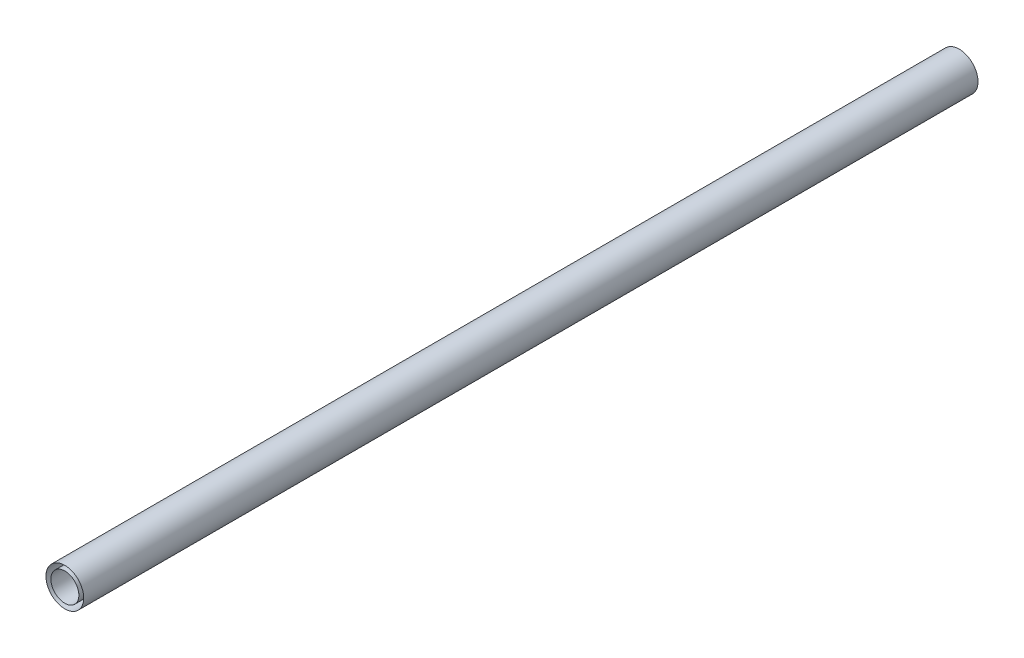
from build123d import *

# Parameters (mm, degrees)
SKETCH1_R           = 95
SKETCH1_R_2         = 94.975
BOSS_EXTRUDE1_DEPTH = 4500
SKETCH2_R           = 70.5
SKETCH2_R_2         = 70.475
BOSS_EXTRUDE2_DEPTH = 4500


with BuildPart() as part:
    # Sketch1 → Boss-Extrude1 (new body)
    with BuildSketch(Plane.XY):
        Circle(SKETCH1_R)
        Circle(SKETCH1_R_2, mode=Mode.SUBTRACT)
    extrude(amount=BOSS_EXTRUDE1_DEPTH)


with BuildPart() as body_2:
    # Sketch2 → Boss-Extrude2 (new body)
    with BuildSketch(Plane.XY):
        Circle(SKETCH2_R)
        Circle(SKETCH2_R_2, mode=Mode.SUBTRACT)
    extrude(amount=BOSS_EXTRUDE2_DEPTH)


solid = Compound([part.part, body_2.part])
